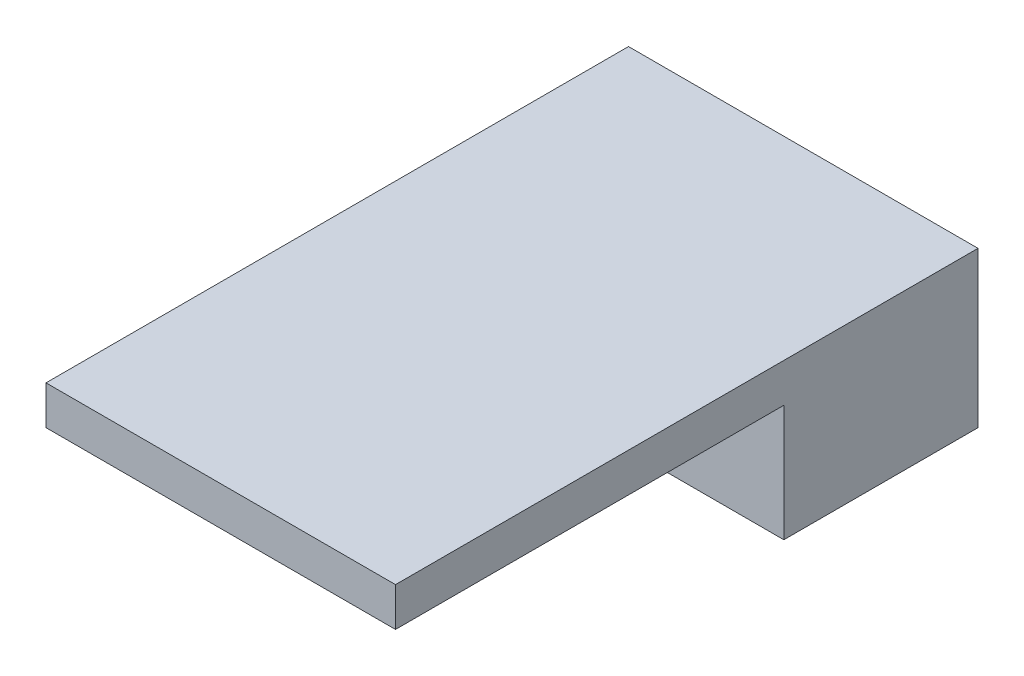
SolidWorks part; units mm, degrees
ref_plane "前视基准面" through (0, 0, 0) normal (0, 0, 1) x (1, 0, 0)
ref_plane "上视基准面" through (0, 0, 0) normal (0, 1, 0) x (1, 0, 0)
ref_plane "右视基准面" through (0, 0, 0) normal (1, 0, 0) x (0, 0, -1)
sketch "草图1" plane through (0, 0, 0) normal (0, 0, 1) x (1, 0, 0)
  line L1 (-9, -4) -> (9, -4)
  line L2 (-9, -4) -> (-9, 4)
  line L3 (-9, 4) -> (9, 4)
  line L4 (9, -4) -> (9, 4)
  line L5 (-9, -4) -> (9, 4) construction
  line L6 (-9, 4) -> (9, -4) construction
  point P0 (0, 0)
  dimension "D1" = 18
  dimension "D2" = 8
extrude "凸台-拉伸1" add sketch "草图1" along normal blind 10
sketch "草图2" plane through (0, 0, 10) normal (0, 0, 1) x (1, 0, 0)
  line L0 (9, -4) -> (9, 4) construction
  line L1 (-9, 4) -> (9, 4)
  line L2 (-9, 4) -> (-9, 2)
  line L3 (-9, 2) -> (9, 2)
  line L4 (9, 4) -> (9, 2)
  dimension "D1" = 2
extrude "凸台-拉伸2" add sketch "草图2" along normal blind 20
hole_wizard "M3 螺纹孔1" positions "3D草图1" profile "草图3" tap size "M3" standard "GB"
sketch3d "3D草图1"
  line L0 (-9, -4, 0) -> (9, -4, 0) construction
  line L1 (9, -4, 0) -> (9, 4, 0) construction
  point P0 (5, 0, 0)
  dimension "D1" = 4
  dimension "D2" = 4
sketch "草图3" plane through (5, 0, 0) normal (1, 0, 0) x (0, 1, 0)
  line L0 (0, 0) -> (0, 7.2511)
  line L1 (0, 7.2511) -> (1.25, 6.5)
  line L2 (1.25, 6.5) -> (1.25, 0.275)
  line L3 (1.25, 0.275) -> (1.525, 0)
  line L5 (1.525, 0) -> (0, 0)
  line L6 (-1.25, 0.275) -> (-1.525, 0) construction
  line L10 (0, 7.2511) -> (-1.25, 6.5) construction
  line L11 (0, -6.35) -> (0, 107.95) construction
  dimension "螺纹孔钻头直径" = 2.5
  dimension "螺纹孔钻头深度" = 6.5
  dimension "近端锥形沉头孔直径" = 3.05
  dimension "近端锥形沉头孔角度" = 90
  dimension "导头角度" = 118
cosmetic thread "孔螺蚊线1" parameters "D1"=5, "D2"=3
mirror "镜向1" about plane through (0, 0, 0) normal (1, 0, 0) of "M3 螺纹孔1"
